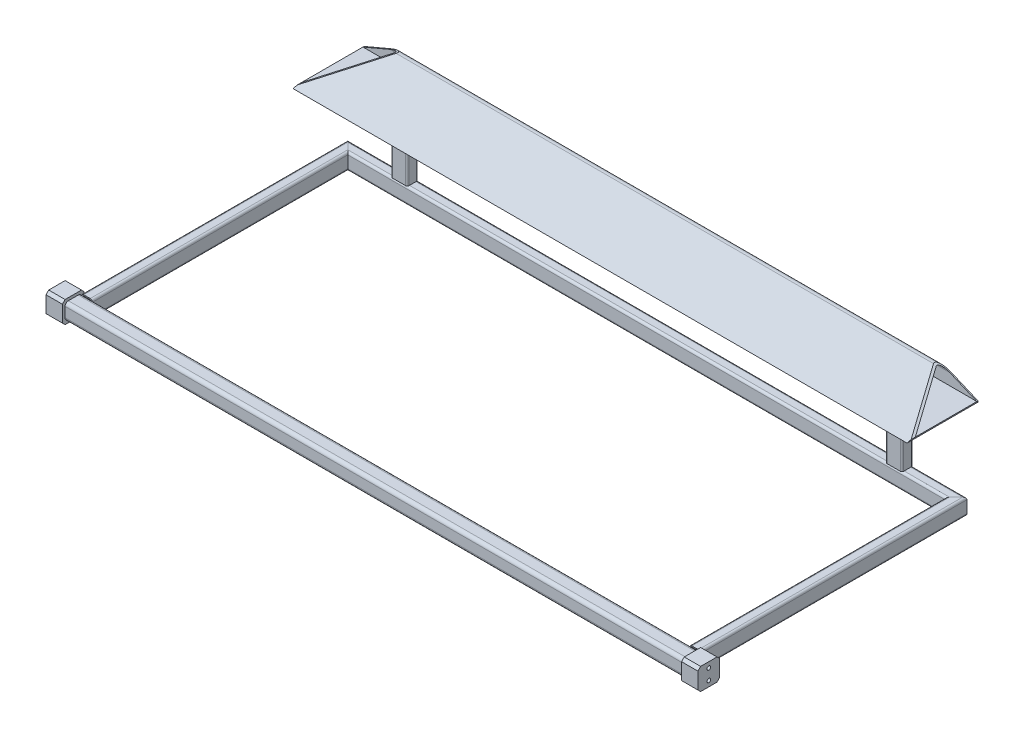
SolidWorks part; units mm, degrees
material "1023 碳钢板 (SS)"
ref_plane "Front Plane" through (0, 0, 0) normal (0, 0, 1) x (1, 0, 0)
ref_plane "Top Plane" through (0, 0, 0) normal (0, 1, 0) x (1, 0, 0)
ref_plane "Right Plane" through (0, 0, 0) normal (1, 0, 0) x (0, 0, -1)
sketch3d "3DSketch1"
  line L0 (0, 0, 0) -> (1134.5, 0, 0)
  dimension "D1" = 1134.5
other "Cold-formed hollow square steel for structures(gb t6728-2002) 30×3(1)"
ref_plane "Plane1" through (0, 0, 0) normal (1, 0, 0) x (0, 0, -1)
sketch "Sketch1" plane through (0, 0, 0) normal (1, 0, 0) x (0, 0, -1)
  line L0 (-9, -12) -> (9, -12)
  line L1 (-12, -9) -> (-12, 9)
  line L2 (9, 12) -> (-9, 12)
  line L3 (12, 9) -> (12, -9)
  line L4 (-9, -15) -> (9, -15)
  line L5 (-15, -9) -> (-15, 9)
  line L6 (9, 15) -> (-9, 15)
  line L7 (15, 9) -> (15, -9)
  arc A0 (15, 9) -> (9, 15) centre (9, 9) ccw
  arc A1 (9, -15) -> (15, -9) centre (9, -9) ccw
  arc A2 (-15, -9) -> (-9, -15) centre (-9, -9) ccw
  arc A3 (-9, 15) -> (-15, 9) centre (-9, 9) ccw
  arc A4 (-9, 12) -> (-12, 9) centre (-9, 9) ccw
  arc A5 (12, 9) -> (9, 12) centre (9, 9) ccw
  arc A6 (9, -12) -> (12, -9) centre (9, -9) ccw
  arc A7 (-12, -9) -> (-9, -12) centre (-9, -9) ccw
  point P0 (-15, 0)
  point P1 (15, 0)
  point P2 (0, 15)
  point P3 (0, -15)
  point P4 (0, 0)
  point P5 (-15, -15)
  point P6 (15, -15)
  point P7 (15, 15)
  point P8 (-15, 15)
  point P33 (0, 0)
  dimension "D1" = 6
  dimension "D2" = 30
  dimension "D3" = 3
sketch3d "3DSketch2"
  line L0 (1124.5106, -0.4598, -14.993) -> (1124.5106, -0.4598, -493)
  line L1 (0, 0, 0) -> (1134.5, 0, 0) construction
  line L2 (9.9894, -0.4598, -14.993) -> (9.9894, -0.4598, -493)
  line L3 (9.9894, -0.4598, -493) -> (1124.5106, -0.4598, -493)
  line L4 (1124.5106, -0.4598, -14.993) -> (9.9894, -0.4598, -14.993) construction
  dimension "D1" = 10
  dimension "D3" = 10
  dimension "D4" = 15
other "Cold-formed hollow rectangular steel for structures(gb t6728-2002) 30×20×2(2)"
ref_plane "Plane2" through (9.9894, -0.4598, -14.993) normal (0, 0, -1) x (1, 0, 0)
sketch "Sketch12" plane through (9.9894, -0.4598, -14.993) normal (0, 0, -1) x (1, 0, 0)
  line L0 (-6, -13) -> (6, -13)
  line L1 (-8, -11) -> (-8, 11)
  line L2 (6, 13) -> (-6, 13)
  line L3 (8, 11) -> (8, -11)
  line L4 (-6, -15) -> (6, -15)
  line L5 (-10, -11) -> (-10, 11)
  line L6 (6, 15) -> (-6, 15)
  line L7 (10, 11) -> (10, -11)
  arc A0 (10, 11) -> (6, 15) centre (6, 11) ccw
  arc A1 (6, -15) -> (10, -11) centre (6, -11) ccw
  arc A2 (-10, -11) -> (-6, -15) centre (-6, -11) ccw
  arc A3 (-6, 15) -> (-10, 11) centre (-6, 11) ccw
  arc A4 (-6, 13) -> (-8, 11) centre (-6, 11) ccw
  arc A5 (8, 11) -> (6, 13) centre (6, 11) ccw
  arc A6 (6, -13) -> (8, -11) centre (6, -11) ccw
  arc A7 (-8, -11) -> (-6, -13) centre (-6, -11) ccw
  point P0 (0, 15)
  point P1 (10, 0)
  point P2 (0, -15)
  point P3 (-10, 0)
  point P4 (-10, 15)
  point P5 (10, 15)
  point P6 (10, -15)
  point P7 (-10, -15)
  point P8 (0, 0)
  point P33 (0, 0)
  dimension "D1" = 30
  dimension "D2" = 20
  dimension "D3" = 2
  dimension "D4" = 4
sketch "Sketch5" plane through (0, 0, 0) normal (-1, 0, 0) x (0, 0, 1)
  line L0 (-20, 15) -> (-15, 20)
  line L1 (15, -20) -> (-15, -20)
  line L2 (20, -15) -> (20, 15)
  line L3 (15, 20) -> (-15, 20)
  line L4 (-20, -15) -> (-20, 15)
  line L5 (20, -20) -> (-20, 20) construction
  line L6 (20, 20) -> (-20, -20) construction
  line L7 (20, 15) -> (15, 20)
  line L8 (-15, -20) -> (-20, -15)
  line L9 (20, -15) -> (15, -20)
  point P0 (0, 0)
  dimension "D1" = 40
extrude "Boss-Extrude1" add sketch "Sketch5" along normal blind 30 separate body
sketch "Sketch6" plane through (-30, 0, 0) normal (-1, 0, 0) x (0, 0, 1)
  line L0 (0, 20) -> (0, -20) construction
  line L1 (15, 20) -> (-15, 20) construction
  line L2 (-15, -20) -> (15, -20) construction
  circle A0 centre (0, 10) radius 1
  circle A1 centre (0, -10) radius 1
  dimension "D1" = 20
  dimension "D2" = 2
  dimension "D3" = 10
extrude "Cut-Extrude1" cut sketch "Sketch6" against normal blind 30
hole_wizard "M8 Tapped Hole1" positions "3DSketch3" profile "Sketch7" tap size "M8" standard "GB"
sketch3d "3DSketch3"
  line L0 (0, 10, 0) -> (-30, 10, 0) construction
  line L1 (0, -10, 0) -> (-30, -10, 0) construction
  point P0 (-30, 10, 0)
  point P4 (-30, -10, 0)
sketch "Sketch7" plane through (-30, 10, 0) normal (0, 1, 0) x (0, 0, 1)
  line L0 (0, 0) -> (0, 32.0429)
  line L1 (0, 32.0429) -> (3.4, 30)
  line L2 (3.4, 30) -> (3.4, 0)
  line L5 (3.4, 0) -> (0, 0)
  line L10 (0, 32.0429) -> (-3.4, 30) construction
  line L11 (0, -6.35) -> (0, 107.95) construction
  dimension "螺纹孔钻头直径" = 6.8
  dimension "螺纹孔钻头深度" = 30
  dimension "导头角度" = 118
cosmetic thread "Hole-Thread1"
cosmetic thread "Hole-Thread2"
ref_plane "Plane3" through (567.25, 0, 0) normal (-1, 0, 0) x (0, 0, 1)
mirror "Mirror1" about plane through (567.25, 0, 0) normal (-1, 0, 0) of "M8 Tapped Hole1", "Cut-Extrude1", "Boss-Extrude1"
sketch "草图12" plane through (0, 0, -503) normal (0, 0, 1) x (1, 0, 0)
  line L0 (189.0592, 0) -> (378.4375, 0) construction
  line L1 (1134.5106, 10.5402) -> (1134.5106, -11.4598) construction
  circle A0 centre (689.5106, 0) radius 1
  circle A1 centre (724.5106, 0) radius 1
  circle A2 centre (759.5106, 0) radius 1
  circle A3 centre (794.5106, 0) radius 1
  dimension "D1" = 2
  dimension "D2" = 35
  dimension "D3" = 35
  dimension "D4" = 35
  dimension "D5" = 340
extrude "Cut-Extrude4" cut sketch "草图12" along normal blind 2
ref_plane "Plane5" through (0, 0, -249) normal (0, 0, -1) x (-1, 0, 0)
sketch "Sketch14" plane through (0, 14.5402, 0) normal (0, 1, 0) x (1, 0, 0)
  line L0 (567.25, -15) -> (567.25, 503) construction
  line L1 (1134.5, -15) -> (0, -15) construction
  line L2 (1134.5106, 503) -> (-0.0106, 503) construction
  line L3 (1114.5106, 483) -> (19.9894, 483) construction
  line L4 (1008.5, 503) -> (1032.5, 503)
  line L5 (1005.5, 500) -> (1005.5, 486)
  line L6 (1008.5, 483) -> (1032.5, 483)
  line L7 (1035.5, 500) -> (1035.5, 486)
  line L8 (1005.5, 503) -> (1035.5, 483) construction
  line L9 (1005.5, 483) -> (1035.5, 503) construction
  line L10 (1033.5, 500) -> (1033.5, 486)
  line L11 (1008.5, 501) -> (1032.5, 501)
  line L12 (1007.5, 500) -> (1007.5, 486)
  line L13 (1008.5, 485) -> (1032.5, 485)
  line L14 (129, 483) -> (99, 503) construction
  line L15 (129, 503) -> (99, 483) construction
  line L16 (126, 485) -> (102, 485)
  line L17 (127, 500) -> (127, 486)
  line L18 (126, 501) -> (102, 501)
  line L19 (101, 500) -> (101, 486)
  line L20 (99, 500) -> (99, 486)
  line L21 (126, 483) -> (102, 483)
  line L22 (129, 500) -> (129, 486)
  line L23 (126, 503) -> (102, 503)
  arc A0 (1005.5, 500) -> (1008.5, 503) centre (1008.5, 500) cw
  arc A1 (1032.5, 503) -> (1035.5, 500) centre (1032.5, 500) cw
  arc A2 (1005.5, 486) -> (1008.5, 483) centre (1008.5, 486) ccw
  arc A3 (1032.5, 483) -> (1035.5, 486) centre (1032.5, 486) ccw
  arc A4 (1032.5, 485) -> (1033.5, 486) centre (1032.5, 486) ccw
  arc A5 (1032.5, 501) -> (1033.5, 500) centre (1032.5, 500) cw
  arc A6 (1007.5, 500) -> (1008.5, 501) centre (1008.5, 500) cw
  arc A7 (1007.5, 486) -> (1008.5, 485) centre (1008.5, 486) ccw
  arc A8 (127, 486) -> (126, 485) centre (126, 486) cw
  arc A9 (127, 500) -> (126, 501) centre (126, 500) ccw
  arc A10 (102, 501) -> (101, 500) centre (102, 500) ccw
  arc A11 (102, 485) -> (101, 486) centre (102, 486) cw
  arc A12 (102, 483) -> (99, 486) centre (102, 486) cw
  arc A13 (129, 486) -> (126, 483) centre (126, 486) cw
  arc A14 (102, 503) -> (99, 500) centre (102, 500) ccw
  arc A15 (129, 500) -> (126, 503) centre (126, 500) ccw
  point P6 (1020.5, 493)
  point P60 (114, 493)
  dimension "D3" = 3
  dimension "D1" = 30
  dimension "D2" = 20
  dimension "D5" = 876.5
  dimension "D4" = 2
extrude "Boss-Extrude2" add sketch "Sketch14" along normal blind 162 separate body
sketch "Sketch15" plane through (567.25, 0, 0) normal (-1, 0, 0) x (0, 0, 1)
  line L0 (-503, 176.5402) -> (-483, 176.5402)
  line L1 (-483, 176.5402) -> (-483, 171.1812)
  line L2 (-483, 171.1812) -> (-503, 176.5402)
  dimension "D1" = 15
extrude "Cut-Extrude6" cut sketch "Sketch15" against normal through all both and the other way through all
hole_wizard "M6 Tapped Hole1" positions "3DSketch4" profile "Sketch16" tap size "M6" standard "GB"
sketch3d "3DSketch4"
  line L0 (794.5106, 0, -501) -> (794.5106, 0, -503) construction
  line L1 (759.5106, 0, -501) -> (759.5106, 0, -503) construction
  line L2 (724.5106, 0, -501) -> (724.5106, 0, -503) construction
  line L3 (689.5106, 0, -501) -> (689.5106, 0, -503) construction
  point P0 (794.5106, 0, -503)
  point P5 (759.5106, 0, -503)
  point P9 (724.5106, 0, -503)
  point P13 (689.5106, 0, -503)
sketch "Sketch16" plane through (794.5106, 0, -503) normal (1, 0, 0) x (0, 1, 0)
  line L0 (0, 0) -> (0, 17)
  line L1 (0, 17) -> (2.5, 15.4978)
  line L2 (2.5, 15.4978) -> (2.5, 0)
  line L5 (2.5, 0) -> (0, 0)
  line L10 (0, 17) -> (-2.5, 15.4978) construction
  line L11 (0, -6.35) -> (0, 107.95) construction
  dimension "螺纹孔钻头直径" = 5
  dimension "螺纹孔钻头深度" = 17
  dimension "导头角度" = 118
cosmetic thread "Hole-Thread7"
cosmetic thread "Hole-Thread8"
cosmetic thread "Hole-Thread9"
cosmetic thread "Hole-Thread10"
sketch "Sketch17" plane through (567.25, 0, 0) normal (-1, 0, 0) x (0, 0, 1)
  line L0 (-413.1915, 152.4761) -> (-517.0875, 180.3149)
  line L1 (-526, 173.4761) -> (-526, 152.4761)
  line L6 (-500, 175.7364) -> (-486, 171.9851) construction
  line L7 (-526, 152.4761) -> (-413.1915, 152.4761)
  line L10 (-503, 176.5402) -> (-503, 14.5402) construction
  line L11 (-398, 150.4761) -> (-516.5698, 182.2468)
  line L12 (-528, 173.4761) -> (-528, 150.4761)
  line L13 (-528, 150.4761) -> (-398, 150.4761)
  arc A0 (-526, 173.4761) -> (-517.0875, 180.3149) centre (-518.9199, 173.4761) cw
  arc A2 (-528, 173.4761) -> (-516.5698, 182.2468) centre (-518.9199, 173.4761) cw
  point P5 (-398.5176, 146.4737)
  point P6 (-515.1556, 177.7268)
  dimension "D2" = 2
  dimension "D1" = 130
  dimension "D3" = 23
  dimension "D4" = 21
extrude "Boss-Extrude3" add sketch "Sketch17" along normal mid plane 1125 separate body
sketch "Sketch20" plane through (0, 0, -528) normal (0, 0, -1) x (-1, 0, 0)
  line L10 (-1129.75, 152.4761) -> (-1044.75, 188.5565)
  line L11 (-1129.75, 173.4761) -> (-1129.75, 150.4761) construction
  line L12 (-1044.75, 188.5565) -> (-1129.75, 188.5565)
  line L13 (-1129.75, 188.5565) -> (-1129.75, 152.4761)
  line L14 (-567.25, 150.4761) -> (-567.25, 284.8633) construction
  line L15 (-4.75, 150.4761) -> (-1129.75, 150.4761) construction
  line L16 (-89.75, 188.5565) -> (-4.75, 188.5565)
  line L17 (-4.75, 152.4761) -> (-89.75, 188.5565)
  line L18 (-4.75, 188.5565) -> (-4.75, 152.4761)
  dimension "D1" = 2
  dimension "D2" = 23
  dimension "D3" = 85
extrude "Cut-Extrude7" cut sketch "Sketch20" against normal blind 373
